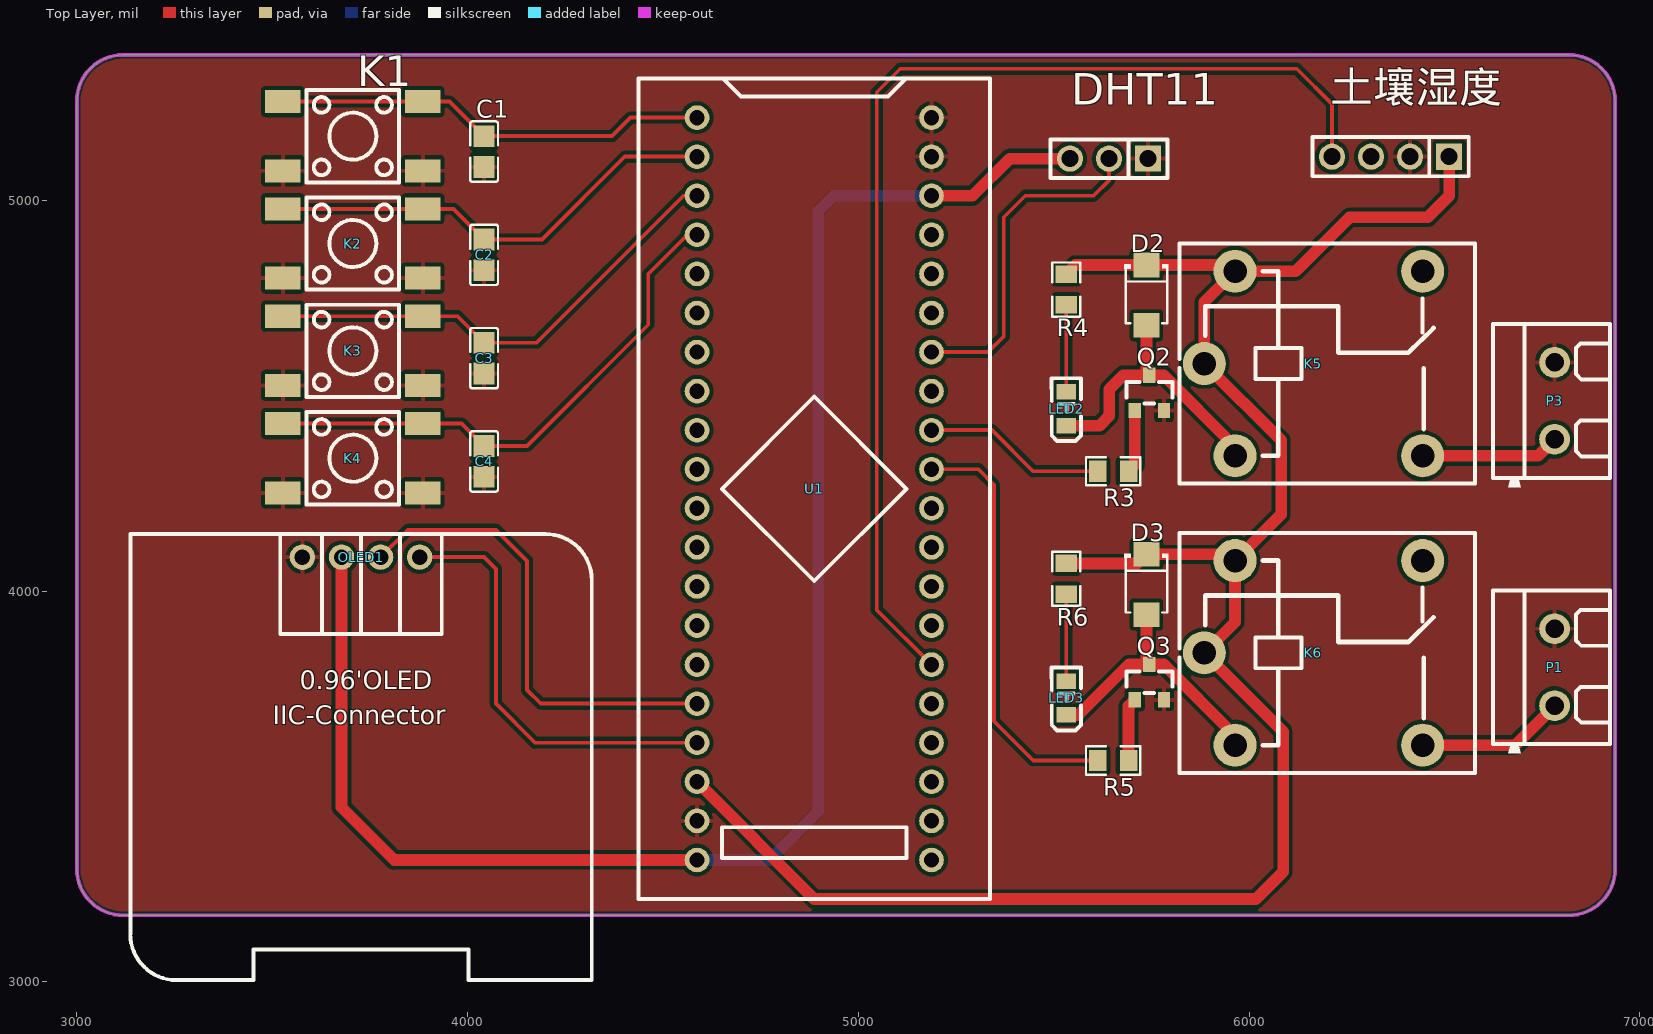
[diagram p0: Top Layer view]
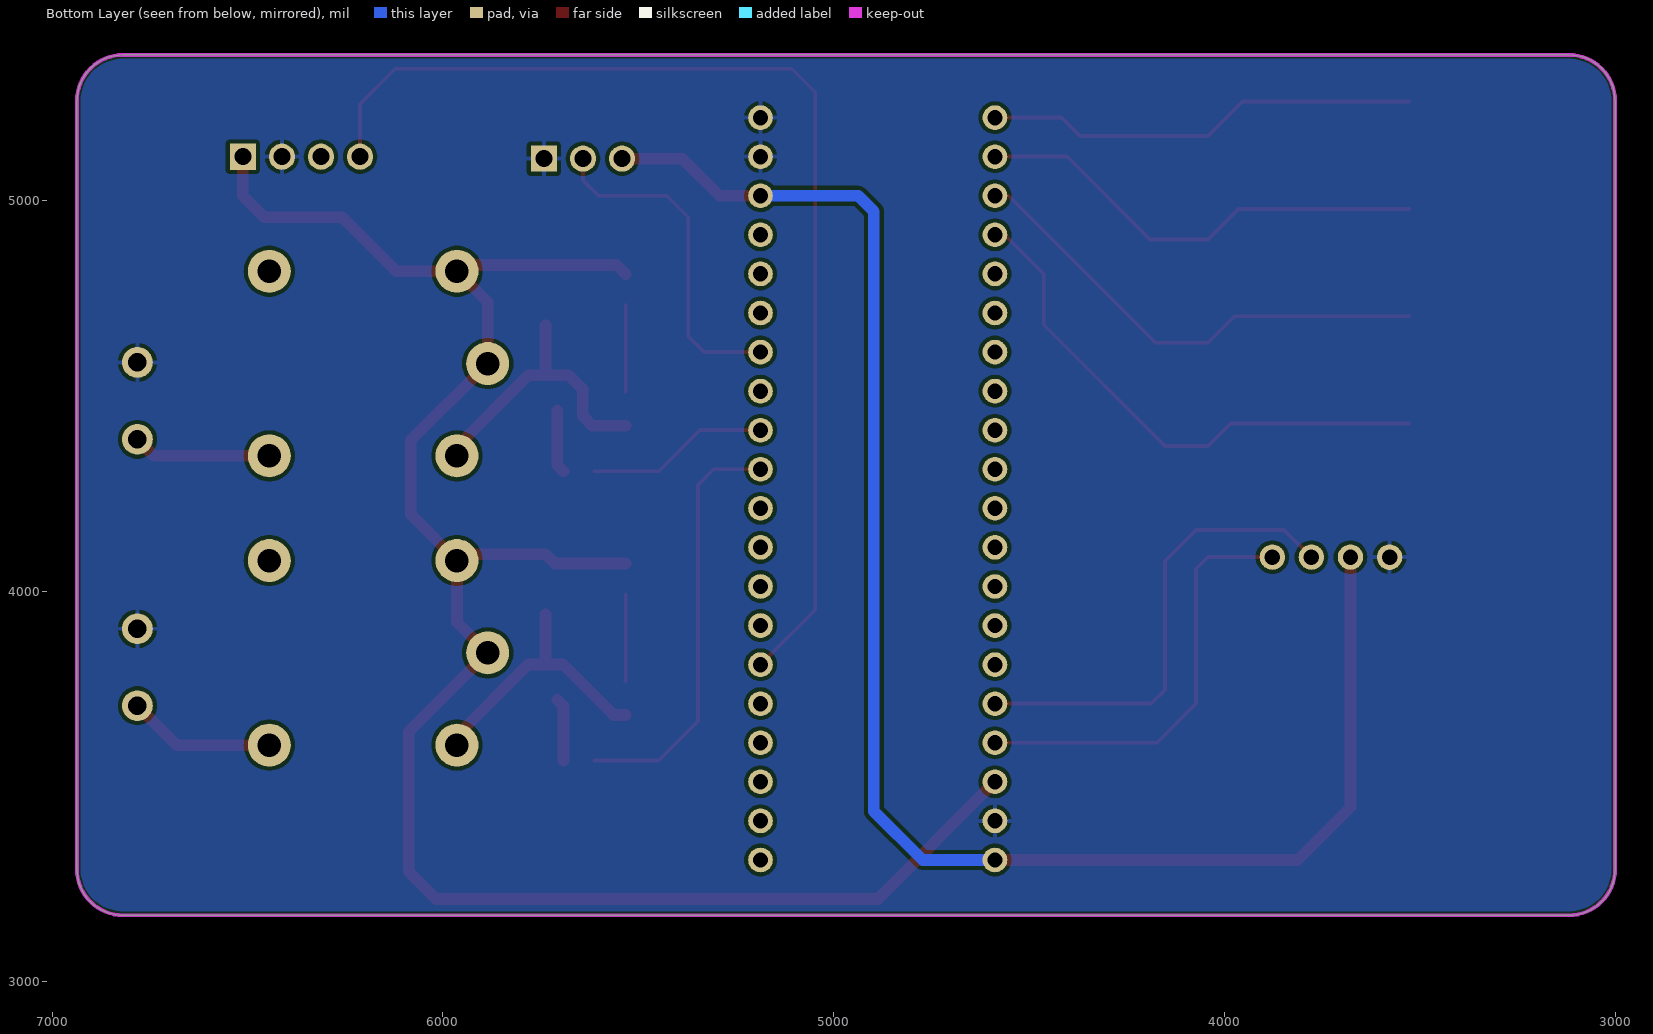
[diagram p1: Bottom Layer view, seen from below]
# Altium PCB MISC51528.pcbdoc
Units mil, origin at the board's own origin, x right, y up, seen from the top; angles counter-clockwise.
Board outline 3937.01 x 2202.01 mil, 2 copper layers (Top Layer, Bottom Layer), stack 62.206 mil thick; 26 components, 45 nets, 111 pads, 0 vias.

## Layer stack, top to bottom
Top Solder Mask Layer: solder mask 0.394, Dk 3.3
Top Layer: signal copper 1.379
Dielectric1: surface 59.449, FR4, Dk 4.5
Bottom Layer: signal copper 1.378
Bottom Solder Mask Layer: solder mask 0.394, Dk 3.3

## Board outline
3118.11,5372.2 ccw(c3118.11,5254.09) 3000,5254.09 3000,3288.3 ccw(c3118.11,3288.3) 3118.11,3170.19 6818.9,3170.19 ccw(c6818.9,3288.3) 6937.01,3288.3 6937.01,5254.09 ccw(c6818.9,5254.09) 6818.9,5372.2 3118.11,5372.2

## Design rules (kind name [scope] priority, off if disabled: settings)
BoardOutlineClearance copperThickness2oz_1 [All] p2 off: genericclearance=7.99 ignorepadtopadclearanceinfootprint=FALSE except(0: Arc-SplitContinuation Track-SplitContinuation SMDPad-SplitContinuation THPad-SplitContinuation Via-SplitContinuation Fill-SplitContinuation Region-SplitContinuation Poly-SplitContinuation Text-SplitContinuation Hole-SplitContinuation; 5.98: Arc-CutoutEdge SMDPad-CutoutEdge THPad-CutoutEdge Via-CutoutEdge Fill-CutoutEdge Region-CutoutEdge Text-CutoutEdge; 6.93: Hole-OutlineEdge Hole-CutoutEdge; 10: Poly-OutlineEdge Poly-CutoutEdge; 11.81: Arc-OutlineEdge Track-OutlineEdge SMDPad-OutlineEdge THPad-OutlineEdge Via-OutlineEdge Fill-OutlineEdge Region-OutlineEdge Text-OutlineEdge Track-CutoutEdge)
BoardOutlineClearance copperThickness1oz_1 [All] p4: genericclearance=4.02 ignorepadtopadclearanceinfootprint=FALSE except(0: Arc-SplitContinuation Track-SplitContinuation SMDPad-SplitContinuation THPad-SplitContinuation Via-SplitContinuation Fill-SplitContinuation Region-SplitContinuation Poly-SplitContinuation Text-SplitContinuation Hole-SplitContinuation; 6: SMDPad-CutoutEdge THPad-CutoutEdge Via-CutoutEdge Fill-CutoutEdge Region-CutoutEdge Text-CutoutEdge; 6.93: Hole-OutlineEdge Hole-CutoutEdge; 10: Poly-OutlineEdge Poly-CutoutEdge; 11.8: Arc-OutlineEdge Track-OutlineEdge SMDPad-OutlineEdge THPad-OutlineEdge Via-OutlineEdge Fill-OutlineEdge Region-OutlineEdge Text-OutlineEdge; 11.81: Arc-CutoutEdge Track-CutoutEdge)
Clearance copperThickness2oz [All] p1 off: gap=7.99 ignorepadtopadclearanceinfootprint=FALSE except(5.98: SMDPad-Track SMDPad-SMDPad THPad-Track SMDPad-THPad THPad-THPad Track-Via SMDPad-Via THPad-Via Via-Via Fill-Track Region-Track Fill-SMDPad Region-SMDPad Fill-THPad Region-THPad Fill-Via Region-Via Fill-Fill Fill-Region Region-Region Arc-Track Arc-SMDPad Arc-THPad Arc-Via Fill-Arc Region-Arc Arc-Arc Text-Track SMDPad-Text Text-THPad Text-Via Fill-Text Region-Text Arc-Text Text-Text; 6.93: Hole-Track Hole-SMDPad Hole-THPad Hole-Via Fill-Hole Region-Hole Hole-Arc Hole-Text; 10: Poly-Track Poly-SMDPad Poly-THPad Poly-Via Poly-Fill Poly-Region Poly-Poly Poly-Arc Poly-Text Poly-Hole)
Clearance copperThickness1oz [All] p3: gap=4.02 ignorepadtopadclearanceinfootprint=FALSE except(5.98: SMDPad-Track SMDPad-SMDPad THPad-Track SMDPad-THPad THPad-THPad Track-Via SMDPad-Via THPad-Via Via-Via Fill-Track Region-Track Fill-SMDPad Region-SMDPad Fill-THPad Region-THPad Fill-Via Region-Via Fill-Fill Fill-Region Region-Region; 6: Arc-Track Arc-SMDPad Arc-THPad Arc-Via Fill-Arc Region-Arc Arc-Arc Text-Track SMDPad-Text Text-THPad Text-Via Fill-Text Region-Text Arc-Text Text-Text; 6.93: Hole-Track Hole-SMDPad Hole-THPad Hole-Via Fill-Hole Region-Hole Hole-Arc Hole-Text; 10: Poly-Track Poly-SMDPad Poly-THPad Poly-Via Poly-Fill Poly-Region Poly-Poly Poly-Arc Poly-Text Poly-Hole)
DiffPairsRouting differentialPair [All] p1: maxlimit=6 minlimit=6 mostfreqgap=6 toplayer_minwidth=5 toplayer_prefwidth=10 toplayer_maxwidth=100 toplayer_mingap=6 toplayer_prefgap=6 toplayer_maxgap=6 bottomlayer_minwidth=5 bottomlayer_prefwidth=10 bottomlayer_maxwidth=100 bottomlayer_mingap=6 bottomlayer_prefgap=6 bottomlayer_maxgap=6 maxuncoupledlength=10
HoleToHoleClearance otherClearance [All] p1: gap=11.81 allowstackedmicrovias=TRUE
Length netLength [All] p1: minlimit=0 maxlimit=0
MatchedLengths netLengthTolerance [All] p1: tolerance=1000
PasteMaskExpansion pasteMaskExpansion [All] p1: expansion=0
PlaneConnect innerPlane [All] p1: planeconnectstyle=Relief reliefexpansion=20 reliefentries=4 reliefconductorwidth=10 reliefairgap=10
PolygonConnect copperRegion [(InNet('GND'))] p1: connectstyle=Relief reliefconductorwidth=10 reliefentries=4 polygonreliefangle="90 Angle" airgapwidth=10 via.connectstyle=Relief via.reliefconductorwidth=10 via.reliefentries=4 via.polygonreliefangle="90 Angle" via.airgapwidth=10
RoutingVias viaSize [All] p1: holewidth=12.01 width=24.02 viastyle="Through Hole" minholewidth=11.81 minwidth=19.68 maxholewidth=248.03 maxwidth=393.7
SolderMaskExpansion solderMaskExpansion [IsVia] p1: expansion=-1000 istentingtop=TRUE
SolderMaskExpansion solderMaskExpansion [All] p2: expansion=2 istentingtop=FALSE
Width copperThickness2oz_2 [All] p1 off: maxlimit=100 minlimit=8 preferedwidth=10
Width copperThickness1oz_2 [All] p2: maxlimit=100 minlimit=5 preferedwidth=10

## Components (designator, comment, footprint, x,y, rotation, side; value= is the part's Value field where it differs from the comment)
C1 "100nF" C0805 4042.28,5124.76 r270 top
C2 "100nF" C0805 4042.28,4860.38 r270 top
C3 "100nF" C0805 4042.28,4595.99 r270 top
C4 "100nF" C0805 4042.28,4331.61 r270 top
D2 "M7F" SMAF_L3.5-W2.6-LS4.7-RD 5737.34,4757.2 r270 top
D3 "M7F" SMAF_L3.5-W2.6-LS4.7-RD 5737.34,4016.8 r270 top
DHT11 "" HDR-TH_3P-P2.54-V-M 5641.59,5106.61 r180 top
K1 "" SW-SMD_4P-L6.0-W6.0-P4.50-LS9.0-2 3706.22,5164.13 r0 top
K2 "" SW-SMD_4P-L6.0-W6.0-P4.50-LS9.0-2 3706.22,4889.39 r0 top
K3 "" SW-SMD_4P-L6.0-W6.0-P4.50-LS9.0-2 3706.22,4614.66 r0 top
K4 "" SW-SMD_4P-L6.0-W6.0-P4.50-LS9.0-2 3706.22,4339.92 r0 top
K5 "SRD-DC5V-SL-C" RELAY-TH_SRD-DCXXV-SL-C 6165,4582.2 r0 top
K6 "SRD-DC5V-SL-C" RELAY-TH_SRD-DCXXV-SL-C 6165,3841.8 r0 top
LED2 "MS-PTV1608NWAF-B02" LED0805-RD_BLUE 5532.48,4466.61 r90 top
LED3 "MS-PTV1608NWAF-B02" LED0805-RD_BLUE 5532.48,3726.21 r90 top
OLED1 "" 0.96OLED_4P 3727.28,4086.61 r0 top
P1 "KF301-2P接线端子" CONN-TH_XY301V-A-5.0-2P 6782,3804.94 r270 top
P3 "KF301-2P接线端子" CONN-TH_XY301V-A-5.0-2P 6782,4486.61 r270 top
Q2 "" S8050_SOT-23 5740,4507.2 r270 top
Q3 "" S8050_SOT-23 5740,3766.8 r270 top
R3 "330" R0805 5652.28,4306.61 r180 top
R4 "10K" R0805 5532.28,4771.61 r90 top
R5 "330" R0805 5652.28,3566.21 r180 top
R6 "10K" R0805 5532.28,4031.21 r90 top
U1 "LCKFB-DKX-STM32F103C8T6" CONN-TH_L53.3-W22.9_STM32F103C8T6-CARD 4887.28,4261.61 r270 top
土壤湿度 "" HDR-TH_4P-P2.54-V-M 6362.28,5111.61 r180 top

## Footprints (in the part's own frame and the unit in brackets; to place one, negate y for a bottom-side part, rotate by r counter-clockwise, add the part's x,y. Pads: shape width x height; smd on the part's side, far side on the other; paste and mask are expansions set on the pad)
0.96OLED_4P [mm]
  round 1.65 hole 1 copper offset 0,0: 1(-3.81,-0.001) 2(-1.27,0.002) 3(1.27,0.002) 4(3.81,0.002)
  silkscreen extent -15,-27.5 15,1.5
C0805 [mm]
  rect 1.41x1.35 smd paste-100 mask+0.051: 1(-1,0) 2(1,0)
  silkscreen extent -1.96,-0.9 1.96,0.9
CONN-TH_L53.3-W22.9_STM32F103C8T6-CARD [mm]
  round 1.6 hole 1: 1(-24.13,-7.62) 2(-21.59,-7.62) 3(-19.05,-7.62) 4(-16.51,-7.62) 5(-13.97,-7.62) 6(-11.43,-7.62) 7(-8.89,-7.62) 8(-6.35,-7.62) 9(-3.81,-7.62) 10(-1.27,-7.62) 11(1.27,-7.62) 12(3.81,-7.62) 13(6.35,-7.62) 14(8.89,-7.62) 15(11.43,-7.62) 16(13.97,-7.62) 17(16.51,-7.62) 18(19.05,-7.62) 19(21.59,-7.62) 20(24.13,-7.62) 21(24.13,7.62) 22(21.59,7.62) 23(19.05,7.62) 24(16.51,7.62) 25(13.97,7.62) 26(11.43,7.62) 27(8.89,7.62) 28(6.35,7.62) 29(3.81,7.62) 30(1.27,7.62) 31(-1.27,7.62) 32(-3.81,7.62) 33(-6.35,7.62) 34(-8.89,7.62) 35(-11.43,7.62) 36(-13.97,7.62) 37(-16.51,7.62) 38(-19.05,7.62) 39(-21.59,7.62) 40(-24.13,7.62)
  silkscreen extent -26.67,-11.43 26.67,11.43
CONN-TH_XY301V-A-5.0-2P [mm]
  round 2 hole 1.2: 1(-2.5,0) 2(2.5,0)
  silkscreen extent -5,-4 5.6,3.6
HDR-TH_3P-P2.54-V-M [mm]
  rect 1.7x1.7 hole 1.1: 1(-2.54,0)
  round 1.7 hole 1.1: 2(0,0) 3(2.54,0)
  silkscreen extent -3.81,-1.25 3.81,1.25
HDR-TH_4P-P2.54-V-M [mm]
  rect 1.7x1.7 hole 1.1: 1(-3.81,0)
  round 1.7 hole 1.1: 2(-1.27,0) 3(1.27,0) 4(3.81,0)
  silkscreen extent -5.08,-1.27 5.08,1.27
LED0805-RD_BLUE [mm]
  rect 1x1.25 smd: 1(-1.1,0) 2(1.1,0)
  silkscreen extent -2.1,-0.95 1.98,0.96
R0805 [mm]
  rect 1.133x1.377 smd paste-100 mask+0.051: 1(-1,0) 2(1,0)
  silkscreen extent -1.76,-0.92 1.76,0.92
RELAY-TH_SRD-DCXXV-SL-C [mil]
  round 110 hole 60: 1(-200.79,-236.22) 2(279.52,-236.2) 3(279.53,236.2) 4(-200.79,236.22) 5(-279.53,0)
  silkscreen extent -342,-307 413,307
S8050_SOT-23 [mm]
  rect 1x0.8 smd paste+0 mask+0.051: 1(1.15,-0.823) 2(1.15,1.077) 3(-1.15,0.127)
  silkscreen extent -0.7,-1.37 0.7,1.63
SMAF_L3.5-W2.6-LS4.7-RD [mm]
  rect 1.6x1.7 smd: 1(-1.96,0) 2(1.96,0)
  silkscreen extent -2.01,-1.43 1.83,1.42
SW-SMD_4P-L6.0-W6.0-P4.50-LS9.0-2 [mm]
  rect 2.3x1.5 smd: 1(-4.55,2.25) 2(4.55,2.25) 3(-4.55,-2.25) 4(4.55,-2.25)
  silkscreen extent -3,-3 3,3

## Nets (pads, with @x,y where several pads share a name; then routed paths per layer and width w, separated by ;. In a path a pad name is that pad's centre, name@x,y a point inside that pad or via, vN(x,y) a via of type N, cw(c..) or ccw(c..) an arc to the next point about the centre after c; other vN are vias at no path point)
$1N24: Q2.1 R3.1 | length 161.9
  Top Layer w30: R3.1 5707.6,4322.56 Q2.1
$1N25: D2.2 K5.1 LED2.1 Q2.3 | length 755.5
  Top Layer w30: LED2.1 5617.45,4423.3 5642.28,4448.13 5642.28,4516.61 5678.15,4552.48 Q2.3 ; D2.2 5737.34,4560.14 Q2.3 ; K5.1 5964.21,4369.69 5781.42,4552.48 Q2.3
$1N26: LED2.2 R4.1 | length 222.4
  Top Layer w10: R4.1 5532.28,4510.12 LED2.2
$1N29: D3.2 K6.1 LED3.1 Q3.3 | length 715.6
  Top Layer w30: LED3.1 5563.57,3682.9 5692.74,3812.07 Q3.3 ; D3.2 5737.34,3819.73 Q3.3 ; K6.1 5964.21,3629.69 5781.82,3812.07 Q3.3
$1N30: LED3.2 R6.1 | length 222.4
  Top Layer w10: R6.1 5532.28,3769.71 LED3.2
$1N32: Q3.1 R5.1 | length 161.9
  Top Layer w30: R5.1 5691.65,3705.58 Q3.1
$1N64: K5.2 P3.2 | length 354.9
  Top Layer w30: K5.2 6739.82,4346 P3.2
$1N121: K6.2 P1.2 | length 379.3
  Top Layer w30: K6.2 6681.08,3605.6 P1.2
+3.3V: DHT11.3 OLED1.2 U1.20 U1.38 | length 4203
  Top Layer w30: OLED1.2 3677.28,3446.61 3812.29,3311.61 U1.20 ; U1.38 5292.28,5011.61 5387.28,5106.61 DHT11.3
  Bottom Layer w30: U1.20 4772.28,3311.61 4897.28,3436.61 4897.28,4971.61 4937.28,5011.61 U1.38
+5V: D2.1 D3.1 K5.4 K5.5 K6.4 K6.5 R4.2 R6.2 U1.18 土壤湿度.1 | length 5093.9
  Top Layer w30: U1.18 4887.28,3211.61 6017.28,3211.61 6087.28,3281.61 6087.28,3639.98 K6.5 5964.21,3920.54 K6.4 ; R6.2 5713.96,4070.58 D3.1 5948.27,4093.96 K6.4 ; R4.2 5555.67,4834.37 D2.1 5948.27,4834.37 K5.4 ; 土壤湿度.1 6512.28,5011.61 6457.28,4956.61 6257.28,4956.61 6119.09,4818.42 K5.4 ; K6.4 6082.28,4196.09 6082.28,4385.39 K5.5 5885.47,4739.68 K5.4
GND: C1.2 C2.2 C3.2 C4.2 DHT11.1 K1.3 K1.4 K2.3 K2.4 K3.3 K3.4 K4.3 K4.4 OLED1.1 P1.1 P3.1 Q2.2 Q3.2 U1.19 U1.39 U1.40 土壤湿度.2
PA0: U1.25
PA1: U1.26 土壤湿度.4 | length 2885.1
  Top Layer w10: U1.26 5047.28,3951.61 5047.28,5276.61 5107.28,5336.61 6122.28,5336.61 6212.28,5246.61 土壤湿度.4
PA2: U1.27
PA3: U1.28
PA4: U1.29
PA5: U1.30
PA6: R5.2 U1.31 | length 1088.8
  Top Layer w10: U1.31 5307.29,4311.61 5347.28,4271.61 5347.28,3666.61 5447.69,3566.21 R5.2
PA7: R3.2 U1.32 | length 469.1
  Top Layer w10: U1.32 5342.29,4411.61 5447.28,4306.61 R3.2
PA8: U1.5
PA9: U1.6
PA10: U1.7
PA11: U1.8
PA12: U1.9
PA15: U1.10
PB0: U1.33
PB1: DHT11.2 U1.34 | length 870.6
  Top Layer w10: U1.34 5332.28,4611.61 5372.28,4651.61 5372.28,4956.61 5427.28,5011.61 5602.28,5011.61 5641.59,5050.92 DHT11.2
PB3: U1.11
PB4: U1.12
PB5: U1.13
PB6: U1.14
PB7: U1.15
PB8: OLED1.3 U1.16 | length 1216.6
  Top Layer w10: OLED1.3 3847.23,4156.61 4072.28,4156.61 4152.28,4076.61 4152.28,3746.61 4187.29,3711.61 U1.16
PB9: OLED1.4 U1.17 | length 1108.9
  Top Layer w10: OLED1.4 4042.23,4086.66 4072.28,4056.61 4072.28,3711.61 4172.29,3611.61 U1.17
PB10: U1.35
PB11: U1.36
PB12: C1.1 K1.1 K1.2 U1.1 | length 1116.5
  Top Layer w10: K1.1 3885.34,5252.72 3953.7,5252.71 C1.1 4369.8,5164.13 4417.28,5211.61 U1.1
PB13: C2.1 K2.1 K2.2 U1.2 | length 1180.3
  Top Layer w10: K2.1 K2.2@3885.34,4977.98 ; K2.2 3964.06,4977.97 C2.1 4190.42,4899.75 4402.28,5111.61 U1.2
PB14: C3.1 K3.1 K3.2 U1.3 | length 1244.1
  Top Layer w10: K3.1 3885.34,4703.24 3974.42,4703.23 C3.1 4176.04,4635.36 4552.28,5011.61 U1.3
PB15: C4.1 K4.1 K4.2 U1.4 | length 1384.1
  Top Layer w10: K4.1 3885.34,4428.5 3984.77,4428.49 C4.1 4151.65,4370.98 4462.28,4681.61 4462.28,4811.61 4562.28,4911.61 U1.4
PC13: U1.22
PC14: U1.23
PC15: U1.24
RES: U1.37
VBAT: U1.21
pads on no net: K5.3 K6.3 土壤湿度.3

## Polygon pours and split planes (outlines as drawn)
GND on Top Layer (solid, remove dead copper, pour order 2): 3118.11,5372.2 ccw(c3118.11,5254.09) 3000,5254.09 3000,3288.3 ccw(c3118.11,3288.3) 3118.11,3170.19 6818.9,3170.19 ccw(c6818.9,3288.3) 6937.01,3288.3 6937.01,5254.09 ccw(c6818.9,5254.09) 6818.9,5372.2 3118.11,5372.2
GND on Bottom Layer (solid, remove dead copper, pour order 2): 3118.11,5372.2 ccw(c3118.11,5254.09) 3000,5254.09 3000,3288.3 ccw(c3118.11,3288.3) 3118.11,3170.19 6818.9,3170.19 ccw(c6818.9,3288.3) 6937.01,3288.3 6937.01,5254.09 ccw(c6818.9,5254.09) 6818.9,5372.2 3118.11,5372.2

## Keep-outs
Board Outline Layer:
  the board outline again, w10